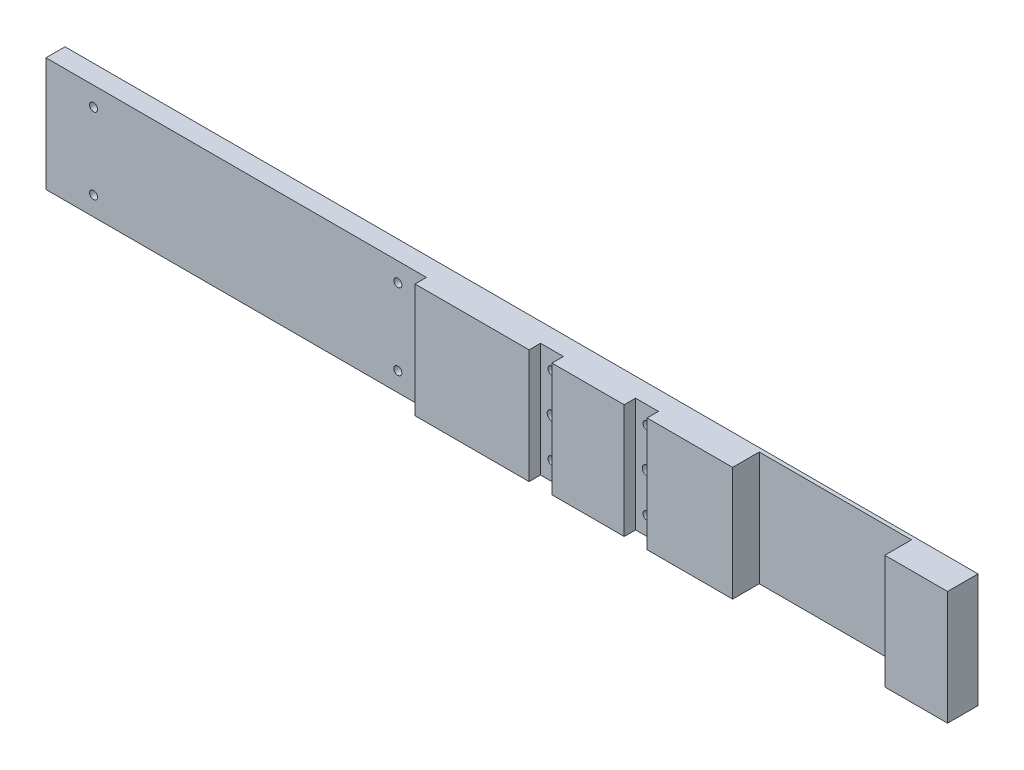
from build123d import *

# Parameters (mm, degrees)
SKETCH_1_W          = 480
SKETCH_1_H          = 60
EXTRUDE_1_DEPTH     = 16
SKETCH_2_W          = 200
SKETCH_2_H          = 60
CUT_EXTRUDE_1_DEPTH = 6
SKETCH_3_W          = 12
SKETCH_3_H          = 60
CUT_EXTRUDE_2_DEPTH = 6
SKETCH_4_R          = 2.1
SKETCH_4_R_2        = 2.5
CUT_EXTRUDE_3_DEPTH = 322.959006961
SKETCH_5_W          = 80
SKETCH_5_H          = 60
CUT_EXTRUDE_4_DEPTH = 14


with BuildPart() as part:
    # 草图1 → 凸台-拉伸1 (new body)
    with BuildSketch(Plane.XY):
        with Locations((80.192307692, -2.163461538)):
            Rectangle(SKETCH_1_W, SKETCH_1_H)
    extrude(amount=EXTRUDE_1_DEPTH)

    # 草图2 → 切除-拉伸1 (cut)
    with BuildSketch(Plane.XY.offset(16)):
        with Locations((-59.807692308, -2.163461538)):
            Rectangle(SKETCH_2_W, SKETCH_2_H)
    extrude(amount=-CUT_EXTRUDE_1_DEPTH, mode=Mode.SUBTRACT)

    # 草图3 → 切除-拉伸2 (cut)
    with BuildSketch(Plane.XY.offset(16)):
        with Locations((106.192307692, -2.163461538)):
            Rectangle(SKETCH_3_W, SKETCH_3_H)
        with Locations((156.192307692, -2.163461538)):
            Rectangle(SKETCH_3_W, SKETCH_3_H)
    extrude(amount=-CUT_EXTRUDE_2_DEPTH, mode=Mode.SUBTRACT)

    # 草图4 → 切除-拉伸3 (cut, through all)
    with BuildSketch(Plane.XY.offset(10)):
        with Locations((-134.807692308, 17.836538462)):
            Circle(SKETCH_4_R)
        with Locations((-134.807692308, -22.163461538)):
            Circle(SKETCH_4_R)
        with Locations((25.192307692, 17.836538462)):
            Circle(SKETCH_4_R)
        with Locations((25.192307692, -22.163461538)):
            Circle(SKETCH_4_R)
        with Locations((106.192307692, 18.336538462)):
            Circle(SKETCH_4_R)
        with Locations((106.192307692, -22.663461538)):
            Circle(SKETCH_4_R)
        with Locations((156.192307692, 18.336538462)):
            Circle(SKETCH_4_R)
        with Locations((156.192307692, -22.663461538)):
            Circle(SKETCH_4_R)
        with Locations((106.192307692, -2.163461538)):
            Circle(SKETCH_4_R_2)
        with Locations((156.192307692, -2.163461538)):
            Circle(SKETCH_4_R_2)
    extrude(amount=-CUT_EXTRUDE_3_DEPTH, mode=Mode.SUBTRACT)

    # 草图5 → 切除-拉伸4 (cut)
    with BuildSketch(Plane.XY.offset(16)):
        with Locations((247.192307692, -2.163461538)):
            Rectangle(SKETCH_5_W, SKETCH_5_H)
    extrude(amount=-CUT_EXTRUDE_4_DEPTH, mode=Mode.SUBTRACT)


solid = part.part
